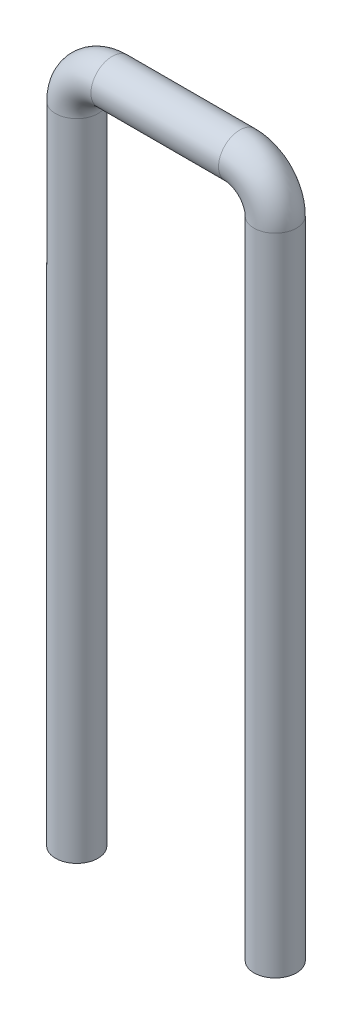
from build123d import *

# Parameters (mm, degrees)
SKETCH_2_R = 3


with BuildPart() as part:
    # 扫描1: sweep along a path in 草图1
    with BuildLine(Plane.XY) as sweep_1_path:
        Line((-14, 0), (-14, 91))
        ThreePointArc((-14, 91), (-12.535533906, 94.535533906), (-9, 96))
        Line((-9, 96), (9, 96))
        ThreePointArc((9, 96), (12.535533906, 94.535533906), (14, 91))
        Line((14, 91), (14, 0))
    # 草图2 → 扫描1 (sweep)
    with BuildSketch(Plane(origin=(0, 0, 0), x_dir=(1, 0, 0), z_dir=(0, 1, 0))):
        with Locations((-14, 0)):
            Circle(SKETCH_2_R)
    sweep(path=sweep_1_path.line)


solid = part.part
